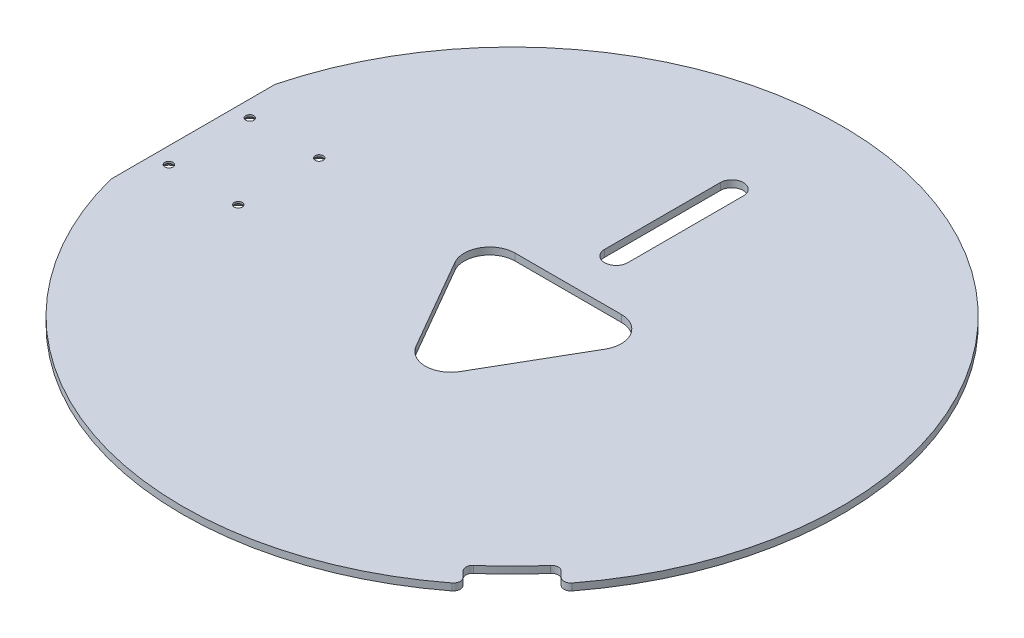
from build123d import *

# Parameters (mm, degrees)
SKETCH1_R           = 142.5
BOSS_EXTRUDE1_DEPTH = 3
SKETCH3_R           = 11
CUT_EXTRUDE1_DEPTH  = 10
CIRPATTERN1_COUNT   = 3
CUT_EXTRUDE2_DEPTH  = 10
CUT_EXTRUDE3_DEPTH  = 10
CUT_EXTRUDE6_START  = -10
CUT_EXTRUDE6_DEPTH  = 10
FILLET1_R           = 3
SKETCH7_W           = 9
SKETCH7_H           = 120
CUT_EXTRUDE7_DEPTH  = 10
SKETCH8_R           = 1.75
CUT_EXTRUDE8_DEPTH  = 10
CHAMFER1_SIZE       = 2.2


with BuildPart() as part:
    # Sketch1 → Boss-Extrude1 (new body)
    with BuildSketch(Plane(origin=(0, 0, 0), x_dir=(1, 0, 0), z_dir=(0, 1, 0))):
        with Locations(Location((0, 0, 0), (0, 0, 270))):
            Circle(SKETCH1_R)
    extrude(amount=BOSS_EXTRUDE1_DEPTH)

    # Sketch3 → Cut-Extrude1 (cut)
    with BuildSketch(Plane(origin=(0, 3, 0), x_dir=(1, 0, 0), z_dir=(0, 1, 0))):
        with Locations(Location((0, -26.5, 0), (0, 0, 270))):
            Circle(SKETCH3_R)
    cut_extrude1 = extrude(amount=-CUT_EXTRUDE1_DEPTH, mode=Mode.SUBTRACT)

    # CirPattern1: Cut-Extrude1 ×3 about axis
    cirpattern1_axis = Axis((0, 0, 0), (0, 1, 0))
    for i in range(1, CIRPATTERN1_COUNT):
        add(cut_extrude1.rotate(cirpattern1_axis, i * 360 / CIRPATTERN1_COUNT), mode=Mode.SUBTRACT)

    # Sketch4 → Cut-Extrude2 (cut)
    with BuildSketch(Plane(origin=(0, 3, 0), x_dir=(1, 0, 0), z_dir=(0, 1, 0))):
        with BuildLine():
            Line((-32.475952642, 7.75), (-9.526279442, -32))
            ThreePointArc((-9.526279442, -32), (0, -37.5), (9.526279442, -32))
            Line((9.526279442, -32), (32.475952642, 7.75))
            ThreePointArc((32.475952642, 7.75), (32.475952642, 18.75), (22.9496732, 24.25))
            Line((22.9496732, 24.25), (-22.9496732, 24.25))
            ThreePointArc((-22.9496732, 24.25), (-32.475952642, 18.75), (-32.475952642, 7.75))
        make_face()
    extrude(amount=-CUT_EXTRUDE2_DEPTH, mode=Mode.SUBTRACT)

    # Sketch5 → Cut-Extrude3 (cut)
    with BuildSketch(Plane(origin=(0, 3, 0), x_dir=(1, 0, 0), z_dir=(0, 1, 0))):
        with BuildLine():
            Line((-5, 45), (-5, 95))
            ThreePointArc((-5, 95), (0, 100), (5, 95))
            Line((5, 95), (5, 45))
            ThreePointArc((5, 45), (0, 40), (-5, 45))
        make_face()
    extrude(amount=-CUT_EXTRUDE3_DEPTH, mode=Mode.SUBTRACT)

    # Sketch6 → Cut-Extrude6 (cut)
    with BuildSketch(Plane(origin=(0, 3, 0), x_dir=(1, 0, 0), z_dir=(0, 1, 0)).offset(CUT_EXTRUDE6_START)):
        with BuildLine():
            Line((89.596317401, -110.809520837), (82.482737092, -103.695940527))
            ThreePointArc((82.482737092, -103.695940527), (93.691648507, -93.691648507), (103.695940527, -82.482737092))
            Line((103.695940527, -82.482737092), (110.809520837, -89.596317401))
            ThreePointArc((110.809520837, -89.596317401), (100.762716319, -100.762716319), (89.596317401, -110.809520837))
        make_face()
    extrude(amount=CUT_EXTRUDE6_DEPTH, mode=Mode.SUBTRACT)

    # Fillet1
    fillet1_edges = [part.edges().sort_by_distance(p)[0] for p in [
        (82.482737092, 1.5, 103.695940527),
        (103.695940527, 1.5, 82.482737092),
        (110.809520837, 1.5, 89.596317401),
        (89.596317401, 1.5, 110.809520837),
    ]]
    fillet(fillet1_edges, radius=FILLET1_R)

    # Sketch7 → Cut-Extrude7 (cut)
    with BuildSketch(Plane(origin=(0, 3, 0), x_dir=(1, 0, 0), z_dir=(0, 1, 0))):
        with Locations((-142.5, 0)):
            Rectangle(SKETCH7_W, SKETCH7_H)
    extrude(amount=-CUT_EXTRUDE7_DEPTH, mode=Mode.SUBTRACT)

    # Sketch8 → Cut-Extrude8 (cut)
    with BuildSketch(Plane(origin=(0, 3, 0), x_dir=(1, 0, 0), z_dir=(0, 1, 0))):
        with Locations(Location((-130.892369907, 17.5, 0), (0, 0, 270))):
            Circle(SKETCH8_R)
        with Locations(Location((-100.892369907, 17.5, 0), (0, 0, 270))):
            Circle(SKETCH8_R)
        with Locations(Location((-130.892369907, -17.5, 0), (0, 0, 270))):
            Circle(SKETCH8_R)
        with Locations(Location((-100.892369907, -17.5, 0), (0, 0, 270))):
            Circle(SKETCH8_R)
    extrude(amount=-CUT_EXTRUDE8_DEPTH, mode=Mode.SUBTRACT)

    # Chamfer1
    chamfer1_edges = [part.edges().sort_by_distance(p)[0] for p in [
        (-130.892369907, 0, -19.25),
        (-100.892369907, 0, -19.25),
        (-130.892369907, 0, 15.75),
        (-100.892369907, 0, 15.75),
    ]]
    chamfer(chamfer1_edges, length=CHAMFER1_SIZE)


solid = part.part
